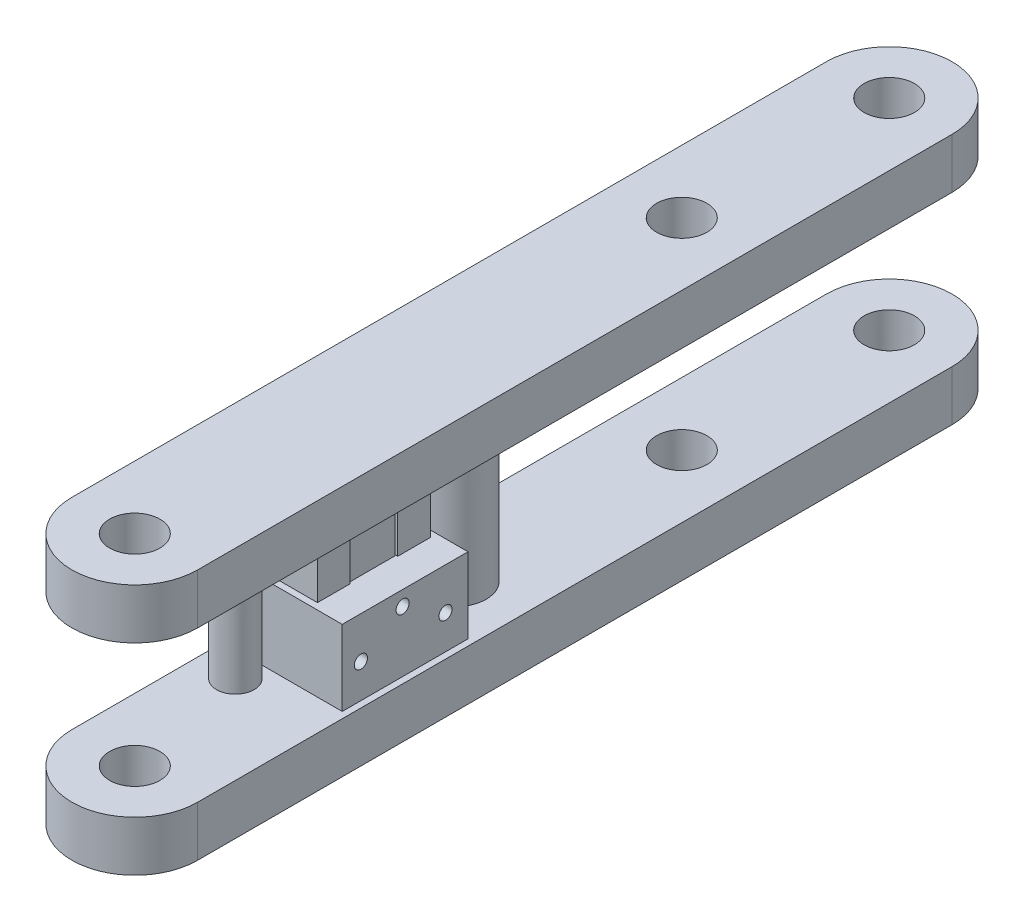
from build123d import *

# Parameters (mm, degrees)
BOSS_EXTRUDE1_DEPTH     = 20
SKETCH2_R               = 2
CUT_EXTRUDE1_DEPTH      = 69.190908485
CUT_EXTRUDE2_DEPTH      = 69.738635424
CUT_EXTRUDE2_DEPTH_BACK = 69.738635424
SKETCH3_W               = 70
SKETCH3_H               = 12
CUT_EXTRUDE3_DEPTH      = 69.190908485
CUT_EXTRUDE3_DEPTH_BACK = 69.190908485
SKETCH4_R               = 2
SKETCH5_R               = 2.5
BOSS_EXTRUDE2_DEPTH     = 16
SKETCH6_R               = 1.5
BOSS_EXTRUDE3_DEPTH     = 16
BOSS_EXTRUDE4_START     = -16
BOSS_EXTRUDE4_DEPTH     = 6
CUT_EXTRUDE4_DEPTH      = 69.667677986
CUT_EXTRUDE4_DEPTH_BACK = 69.667677986
SKETCH8_R               = 0.52328701
SKETCH9_W               = 3.261997226
SKETCH9_H               = 3.598658034
BOSS_EXTRUDE5_DEPTH     = 4
SKETCH10_W              = 3.703262865
SKETCH10_H              = 2.596843015
BOSS_EXTRUDE6_DEPTH     = 6


with BuildPart() as part:
    # Sketch1 → Boss-Extrude1 (new body)
    with BuildSketch(Plane(origin=(0, 0, 0), x_dir=(1, 0, 0), z_dir=(0, 1, 0))):
        with BuildLine():
            Line((-5, 0), (-5, -60))
            ThreePointArc((-5, -60), (0, -65), (5, -60))
            Line((5, -60), (5, 0))
            ThreePointArc((5, 0), (0, 5), (-5, 0))
        make_face()
    extrude(amount=BOSS_EXTRUDE1_DEPTH)

    # Sketch2 → Cut-Extrude1 (cut, through all)
    with BuildSketch(Plane(origin=(0, 20, 0), x_dir=(1, 0, 0), z_dir=(0, 1, 0))):
        with Locations(Location((0, 0, 0), (0, 0, 270))):
            Circle(SKETCH2_R)
        with Locations(Location((0, -16.5, 0), (0, 0, 270))):
            Circle(SKETCH2_R)
    extrude(amount=-CUT_EXTRUDE1_DEPTH, mode=Mode.SUBTRACT)

    # Sketch3 → Cut-Extrude2 (cut, two sides: drawn at the far end of the back side and taken through both)
    with BuildSketch(Plane(origin=(5, 0, 0), x_dir=(0, 0, -1), z_dir=(1, 0, 0)).offset(-CUT_EXTRUDE2_DEPTH_BACK)):
        with Locations((-30, 10)):
            Rectangle(SKETCH3_W, SKETCH3_H)
    extrude(amount=CUT_EXTRUDE2_DEPTH + CUT_EXTRUDE2_DEPTH_BACK, mode=Mode.SUBTRACT)


with BuildPart() as cut_extrude2_piece_1:
    # of the separate pieces the step leaves, piece 1, a body of its own (cut_extrude2_pieces)
    add(part.part.solids().sort_by_distance((5, 16, 60))[0])


with BuildPart() as cut_extrude2_piece_2:
    # of the separate pieces the step leaves, piece 2, a body of its own (cut_extrude2_pieces)
    add(part.part.solids().sort_by_distance((5, 0, 60))[0])


with BuildPart() as cut_extrude3_tool:
    # Sketch4 → Cut-Extrude3 (new, two sides: drawn at the far end of the back side and taken through both)
    with BuildSketch(Plane(origin=(0, 20, 0), x_dir=(1, 0, 0), z_dir=(0, 1, 0)).offset(-CUT_EXTRUDE3_DEPTH_BACK)):
        with Locations(Location((0, -60, 0), (0, 0, 270))):
            Circle(SKETCH4_R)
    extrude(amount=CUT_EXTRUDE3_DEPTH + CUT_EXTRUDE3_DEPTH_BACK)


with BuildPart() as cut_extrude2_piece_1_1:
    add(cut_extrude2_piece_1.part)

    # Cut-Extrude3: cut by cut_extrude3_tool
    add(cut_extrude3_tool.part, mode=Mode.SUBTRACT)



with BuildPart() as cut_extrude2_piece_2_1:
    add(cut_extrude2_piece_2.part)

    # Cut-Extrude3: cut by cut_extrude3_tool
    add(cut_extrude3_tool.part, mode=Mode.SUBTRACT)


with BuildPart() as cut_extrude2_piece_1_2:
    add(cut_extrude2_piece_1_1.part)

    add(cut_extrude2_piece_2_1.part)  # Boss-Extrude2 merges Cut-Extrude2 piece 2
    # Sketch5 → Boss-Extrude2 (add)
    with BuildSketch(Plane(origin=(0, 20, 0), x_dir=(1, 0, 0), z_dir=(0, 1, 0))):
        with Locations(Location((0, -34.552446897, 0), (0, 0, 270))):
            Circle(SKETCH5_R)
    extrude(amount=-BOSS_EXTRUDE2_DEPTH)

    # Sketch6 → Boss-Extrude3 (add)
    with BuildSketch(Plane(origin=(0, 20, 0), x_dir=(1, 0, 0), z_dir=(0, 1, 0))):
        with Locations(Location((-2, -50, 0), (0, 0, 270))):
            Circle(SKETCH6_R)
    extrude(amount=-BOSS_EXTRUDE3_DEPTH)

    # Sketch7 → Boss-Extrude4 (add)
    with BuildSketch(Plane(origin=(0, 20, 0), x_dir=(1, 0, 0), z_dir=(0, 1, 0)).offset(BOSS_EXTRUDE4_START)):
        Polygon((4.5, -38), (-4, -38), (-4, -48), (4.5, -48), (4.5, -44), align=None)
    extrude(amount=BOSS_EXTRUDE4_DEPTH)

    # Sketch8 → Cut-Extrude4 (cut, two sides: drawn at the far end of the back side and taken through both)
    with BuildSketch(Plane(origin=(4.5, 0, 0), x_dir=(0, 0, -1), z_dir=(1, 0, 0)).offset(-CUT_EXTRUDE4_DEPTH_BACK)):
        with Locations((-39.788503734, 6.691891051)):
            Circle(SKETCH8_R)
        with Locations((-46.515921266, 6.691891051)):
            Circle(SKETCH8_R)
        with Locations((-43.19958868, 8.823819142)):
            Circle(SKETCH8_R)
    extrude(amount=CUT_EXTRUDE4_DEPTH + CUT_EXTRUDE4_DEPTH_BACK, mode=Mode.SUBTRACT)

    # Sketch9 → Boss-Extrude5 (add)
    with BuildSketch(Plane(origin=(0, 10, 0), x_dir=(1, 0, 0), z_dir=(0, 1, 0))):
        with Locations((0.25, -43)):
            Rectangle(SKETCH9_W, SKETCH9_H)
    extrude(amount=BOSS_EXTRUDE5_DEPTH)

    # Sketch10 → Boss-Extrude6 (add)
    with BuildSketch(Plane(origin=(0, 10, 0), x_dir=(1, 0, 0), z_dir=(0, 1, 0))):
        with Locations((0.168234256, -39.807752572)):
            Rectangle(SKETCH10_W, SKETCH10_H)
        with Locations((0.168234256, -46.192247429)):
            Rectangle(SKETCH10_W, SKETCH10_H)
    extrude(amount=BOSS_EXTRUDE6_DEPTH)


solid = cut_extrude2_piece_1_2.part
